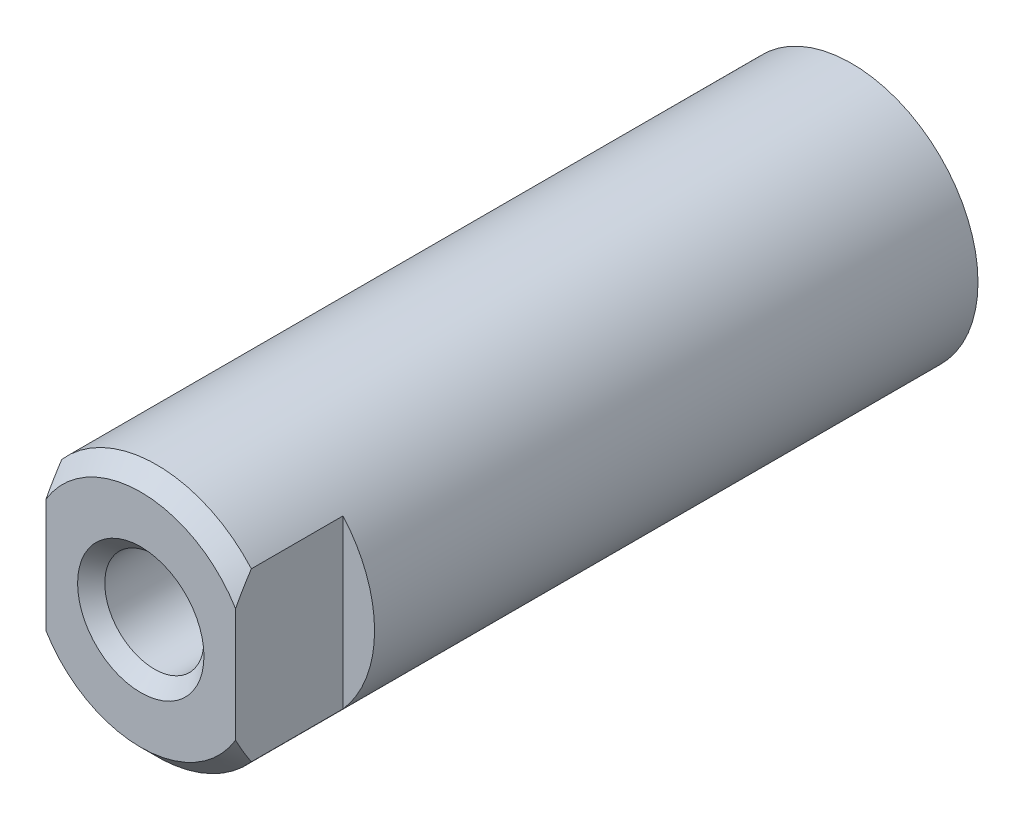
from build123d import *

# Parameters (mm, degrees)
CUT_EXTRUDE_1_DEPTH = 3.4


with BuildPart() as part:
    # 草图1 → 旋转1 (revolve)
    with BuildSketch(Plane(origin=(0, 0, 0), x_dir=(0, 0, -1), z_dir=(1, 0, 0)), mode=Mode.PRIVATE) as revolve_1_sk:
        Polygon((-3.5, 0), (-3.5, 3.5), (-3, 4), (19, 4), (19, 0), align=None)
    revolve(revolve_1_sk.sketch.rotate(Axis((0, 0, -19), (0, 0, 1)), 270), axis=Axis((0, 0, -19), (0, 0, 1)))

    # 草图2 → 切除-拉伸1 (cut)
    with BuildSketch(Plane.XY.offset(3.5)):
        Polygon((-6, -6), (-3, -6), (-3, 6), (3, 6), (3, -6), (6, -6), (6, 8), (-6, 8), align=None)
    extrude(amount=-CUT_EXTRUDE_1_DEPTH, mode=Mode.SUBTRACT)

    # 草图3 → 切除-旋转1 (revolve, cut)
    with BuildSketch(Plane(origin=(0, 0, 0), x_dir=(0, 0, -1), z_dir=(1, 0, 0)), mode=Mode.PRIVATE) as cut_revolve_1_sk:
        Polygon((-4, 0), (-4, 2.5), (-3.07, 1.57), (5, 1.57), (5.906439923, 0), align=None)
    revolve(cut_revolve_1_sk.sketch.rotate(Axis((0, 0, -5.906439923), (0, 0, 1)), 270), axis=Axis((0, 0, -5.906439923), (0, 0, 1)), mode=Mode.SUBTRACT)


solid = part.part
